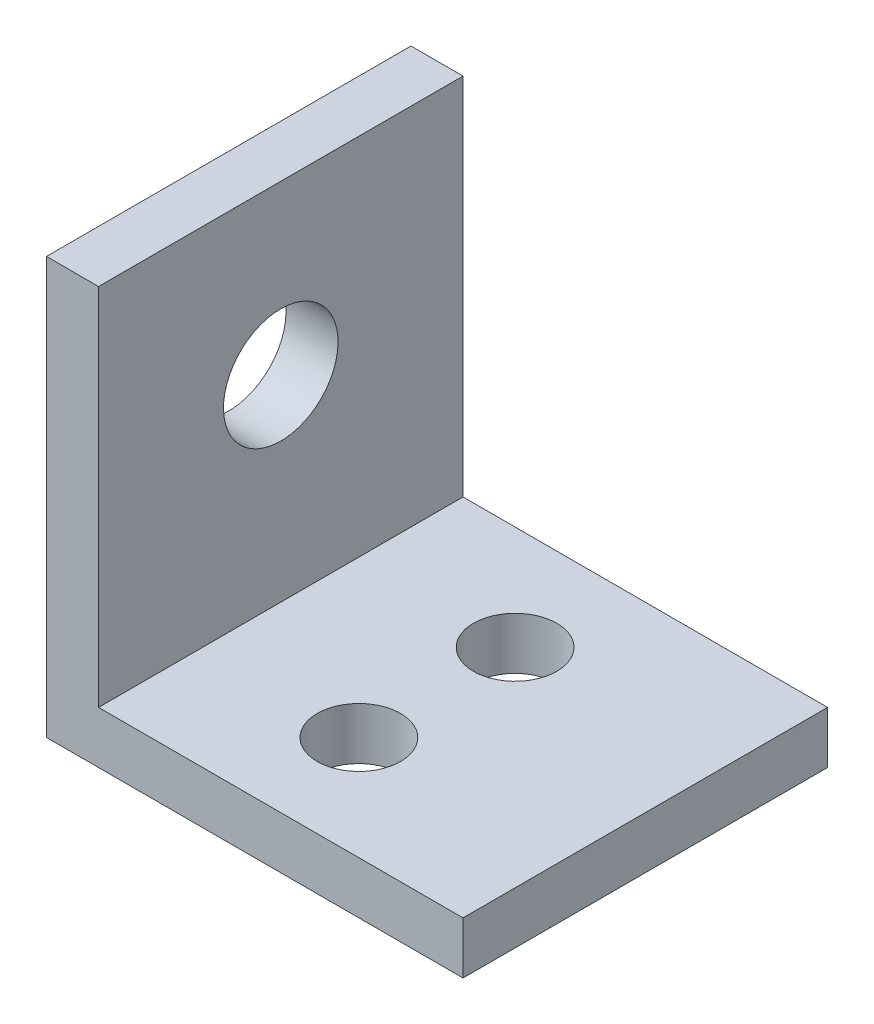
SolidWorks part; units mm, degrees
material "AISI 1015 钢，冷拔 (SS)"
ref_plane "Front Plane" through (0, 0, 0) normal (0, 0, 1) x (1, 0, 0)
ref_plane "Top Plane" through (0, 0, 0) normal (0, 1, 0) x (1, 0, 0)
ref_plane "Right Plane" through (0, 0, 0) normal (1, 0, 0) x (0, 0, -1)
other "Configuration Table"
sketch "Sketch1" plane through (0, 0, 0) normal (0, 0, 1) x (1, 0, 0)
  line L0 (0, 0) -> (0, 80)
  line L1 (0, 80) -> (10, 80)
  line L2 (10, 80) -> (10, 10)
  line L3 (10, 10) -> (80, 10)
  line L4 (80, 10) -> (80, 0)
  line L5 (80, 0) -> (0, 0)
  dimension "D1" = 80
  dimension "D2" = 80
  dimension "D3" = 10
  dimension "D4" = 10
extrude "Boss-Extrude1" add sketch "Sketch1" along normal blind 70
sketch "Sketch2" plane through (0, 10, 0) normal (0, 1, 0) x (1, 0, 0)
  line L0 (80, -70) -> (80, 0) construction
  line L1 (80, 0) -> (10, 0) construction
  circle A0 centre (40, -20) radius 8
  circle A1 centre (40, -50) radius 8
  dimension "D1" = 16
  dimension "D2" = 16
  dimension "D3" = 40
  dimension "D4" = 30
  dimension "D5" = 20
extrude "Cut-Extrude1" cut sketch "Sketch2" against normal blind 90
sketch "Sketch3" plane through (10, 0, 0) normal (1, 0, 0) x (0, 0, -1)
  circle A0 centre (-35, 47.7924) radius 11
  dimension "D1" = 22
extrude "Cut-Extrude2" cut sketch "Sketch3" against normal blind 90
